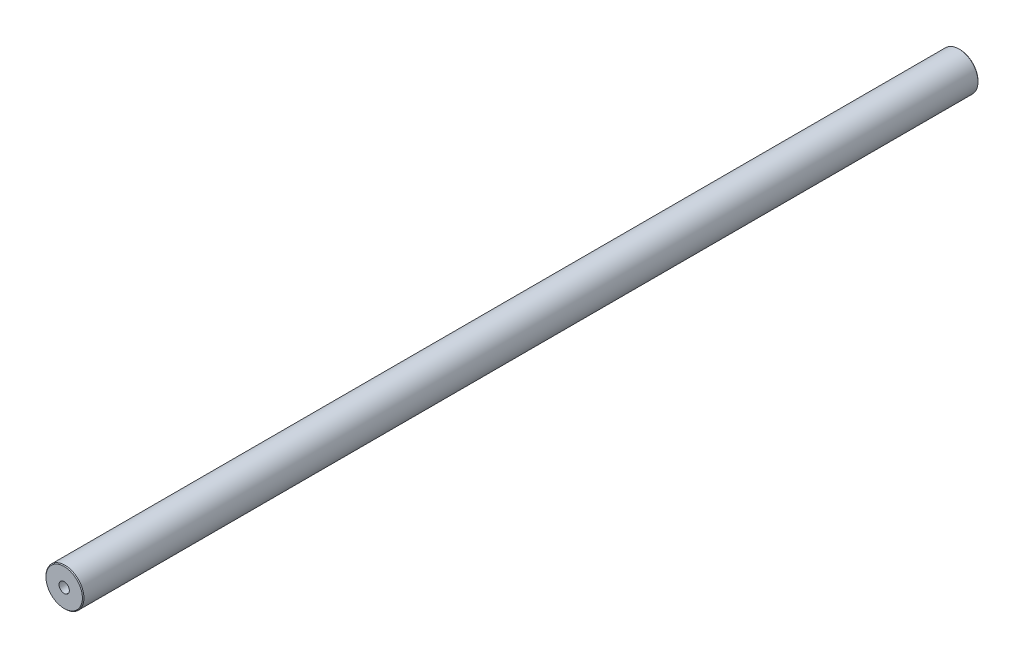
from build123d import *

# Parameters (mm, degrees)
SKETCH_1_R             = 12.5
EXTRUDE_1_DEPTH        = 590
HOLE_WIZARD_M8_1_D     = 6.8
HOLE_WIZARD_M8_1_DEPTH = 19.75
HOLE_WIZARD_M8_1_TIP   = 2.042926105
HOLE_WIZARD_M8_2_D     = 6.8
HOLE_WIZARD_M8_2_DEPTH = 19.75
HOLE_WIZARD_M8_2_TIP   = 2.042926105
CHAMFER_1_SIZE         = 0.5


with BuildPart() as part:
    # 草图1 → 凸台-拉伸1 (new body)
    with BuildSketch(Plane.XY):
        Circle(SKETCH_1_R)
    extrude(amount=EXTRUDE_1_DEPTH)

    # M8 螺纹孔1
    with Locations(Plane.XY.offset(590)):
        with Locations((0, 0)):
            Hole(HOLE_WIZARD_M8_1_D / 2, depth=HOLE_WIZARD_M8_1_DEPTH)
            with Locations((0, 0, -(HOLE_WIZARD_M8_1_DEPTH + HOLE_WIZARD_M8_1_TIP / 2))):  # 118° drill point
                Cone(0, HOLE_WIZARD_M8_1_D / 2, HOLE_WIZARD_M8_1_TIP, mode=Mode.SUBTRACT)

    # M8 螺纹孔2
    with Locations(Plane(origin=(0, 0, 0), x_dir=(-1, 0, 0), z_dir=(0, 0, -1))):
        with Locations((0, 0)):
            Hole(HOLE_WIZARD_M8_2_D / 2, depth=HOLE_WIZARD_M8_2_DEPTH)
            with Locations((0, 0, -(HOLE_WIZARD_M8_2_DEPTH + HOLE_WIZARD_M8_2_TIP / 2))):  # 118° drill point
                Cone(0, HOLE_WIZARD_M8_2_D / 2, HOLE_WIZARD_M8_2_TIP, mode=Mode.SUBTRACT)

    # 倒角1
    chamfer_1_edges = [part.edges().sort_by_distance(p)[0] for p in [
        (-3.4, 0, 0),
        (-12.5, 0, 0),
        (-12.5, 0, 590),
    ]]
    chamfer(chamfer_1_edges, length=CHAMFER_1_SIZE)


solid = part.part
